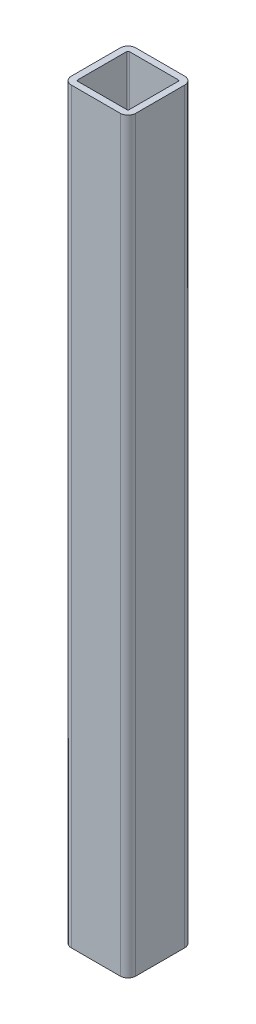
from build123d import *

# Parameters (mm, degrees)
EXTRUDE_1_DEPTH = 580


with BuildPart() as part:
    # 草图1 → 凸台-拉伸1 (new body)
    with BuildSketch(Plane(origin=(0, 0, 0), x_dir=(1, 0, 0), z_dir=(0, 1, 0))):
        with BuildLine():
            Line((-19, -12.278106509), (19, -12.278106509))
            ThreePointArc((19, -12.278106509), (23.242640687, -10.520747196), (25, -6.278106509))
            Line((25, -6.278106509), (25, 31.721893491))
            ThreePointArc((25, 31.721893491), (23.242640687, 35.964534178), (19, 37.721893491))
            Line((19, 37.721893491), (-19, 37.721893491))
            ThreePointArc((-19, 37.721893491), (-23.242640687, 35.964534178), (-25, 31.721893491))
            Line((-25, 31.721893491), (-25, -6.278106509))
            ThreePointArc((-25, -6.278106509), (-23.242640687, -10.520747196), (-19, -12.278106509))
        make_face()
        with BuildLine():
            Line((-19, -7.278106509), (19, -7.278106509))
            ThreePointArc((19, -7.278106509), (19.707106781, -6.98521329), (20, -6.278106509))
            Line((20, -6.278106509), (20, 31.721893491))
            ThreePointArc((20, 31.721893491), (19.707106781, 32.429000272), (19, 32.721893491))
            Line((19, 32.721893491), (-19, 32.721893491))
            ThreePointArc((-19, 32.721893491), (-19.707106781, 32.429000272), (-20, 31.721893491))
            Line((-20, 31.721893491), (-20, -6.278106509))
            ThreePointArc((-20, -6.278106509), (-19.707106781, -6.98521329), (-19, -7.278106509))
        make_face(mode=Mode.SUBTRACT)
    extrude(amount=EXTRUDE_1_DEPTH)


solid = part.part
